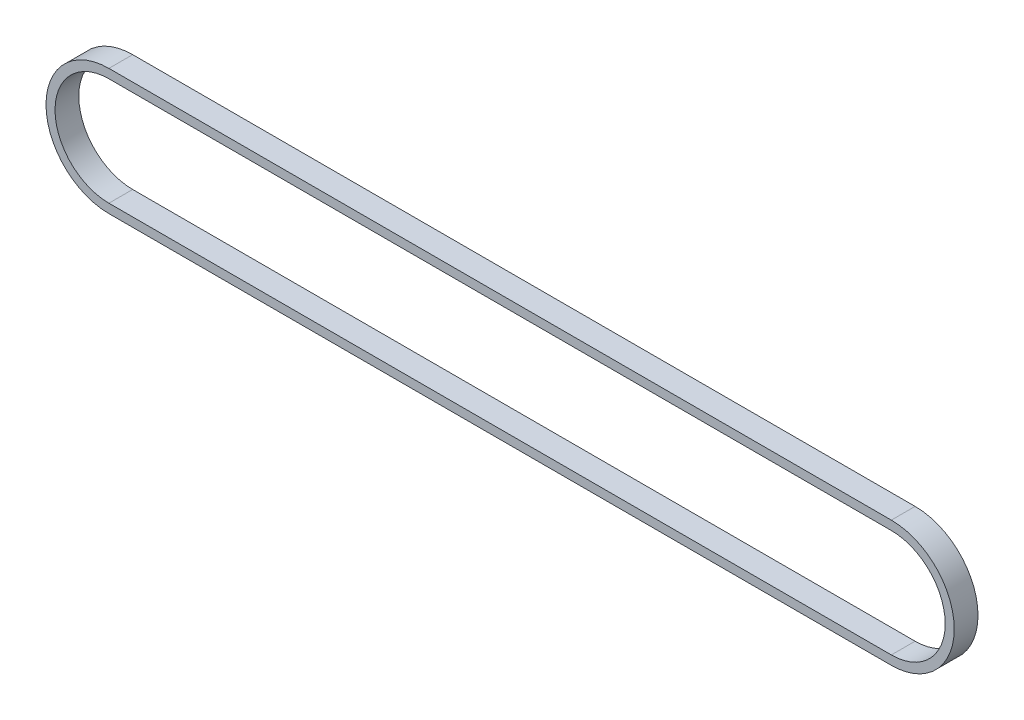
SolidWorks part; units mm, degrees
ref_plane "Front Plane" through (0, 0, 0) normal (0, 0, 1) x (1, 0, 0)
ref_plane "Top Plane" through (0, 0, 0) normal (0, 1, 0) x (1, 0, 0)
ref_plane "Right Plane" through (0, 0, 0) normal (1, 0, 0) x (0, 0, -1)
sketch "Sketch2" plane through (0, 0, 0) normal (0, 0, 1) x (1, 0, 0)
  line L0 (5.5, 0) -> (-5.5, 0) construction
  line L1 (0, 20.9) -> (-260, 20.9)
  line L2 (0, -20.9) -> (-260, -20.9)
  arc A0 (0, -20.9) -> (0, 20.9) centre (0, 0) ccw
  arc A1 (-260, 20.9) -> (-260, -20.9) centre (-260, 0) ccw
  dimension "D1" = 41.8
  dimension "D2" = 41.8
  dimension "D3" = 260
extrude "Boss-Extrude1" add sketch "Sketch2" along normal blind 7.9
shell "Shell1" thickness 3
